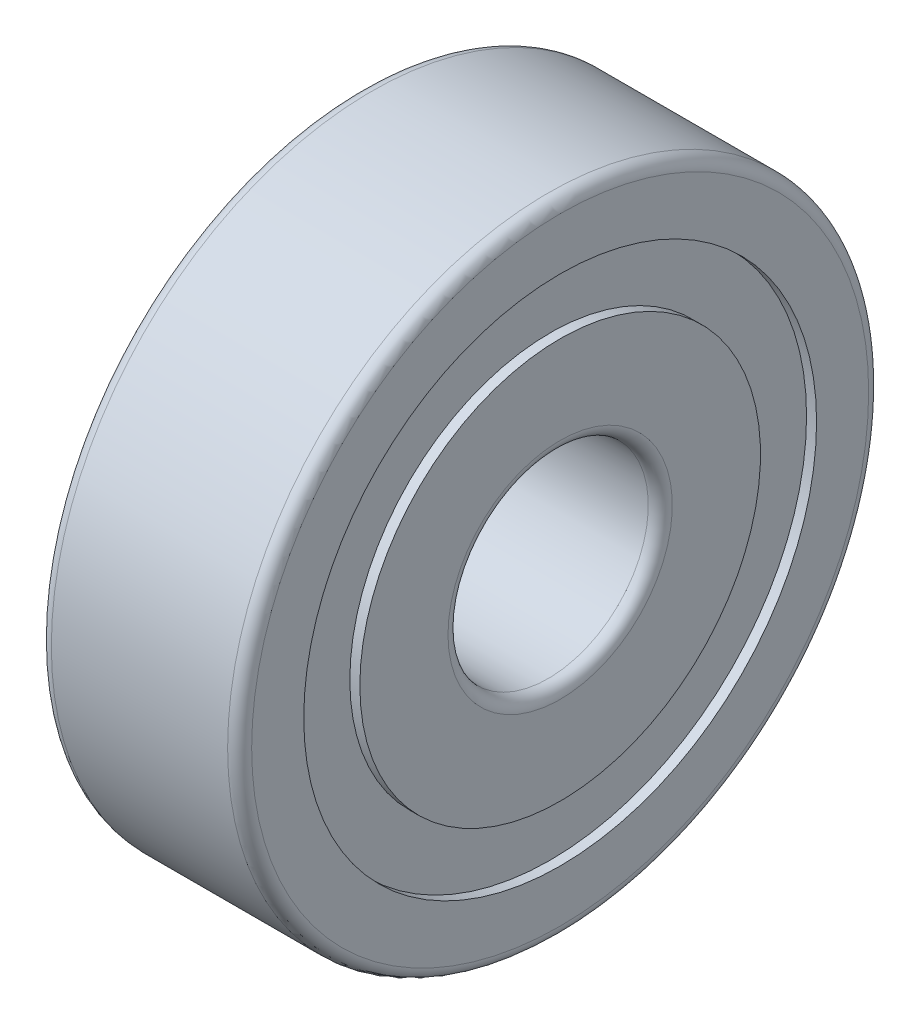
from build123d import *


with BuildPart() as part:
    # 草图1 → 旋转1 (revolve)
    with BuildSketch(Plane.XY, mode=Mode.PRIVATE) as revolve_1_sk:
        with BuildLine():
            Line((-2.5, 7.7), (-2.5, 6.4))
            Line((-2.5, 6.4), (-2.25, 6.4))
            Line((-2.25, 6.4), (-2.25, 5))
            Line((-2.25, 5), (-2.5, 5))
            Line((-2.5, 5), (-2.5, 2.8))
            ThreePointArc((-2.5, 2.8), (-2.412132034, 2.587867966), (-2.2, 2.5))
            Line((-2.2, 2.5), (2.2, 2.5))
            ThreePointArc((2.2, 2.5), (2.412132034, 2.587867966), (2.5, 2.8))
            Line((2.5, 2.8), (2.5, 5))
            Line((2.5, 5), (2.25, 5))
            Line((2.25, 5), (2.25, 6.4))
            Line((2.25, 6.4), (2.5, 6.4))
            Line((2.5, 6.4), (2.5, 7.7))
            ThreePointArc((2.5, 7.7), (2.412132034, 7.912132034), (2.2, 8))
            Line((2.2, 8), (-2.2, 8))
            ThreePointArc((-2.2, 8), (-2.412132034, 7.912132034), (-2.5, 7.7))
        make_face()
    revolve(revolve_1_sk.sketch.rotate(Axis((2.5, 0, 0), (-1, 0, 0)), 270), axis=Axis((2.5, 0, 0), (-1, 0, 0)))


solid = part.part
